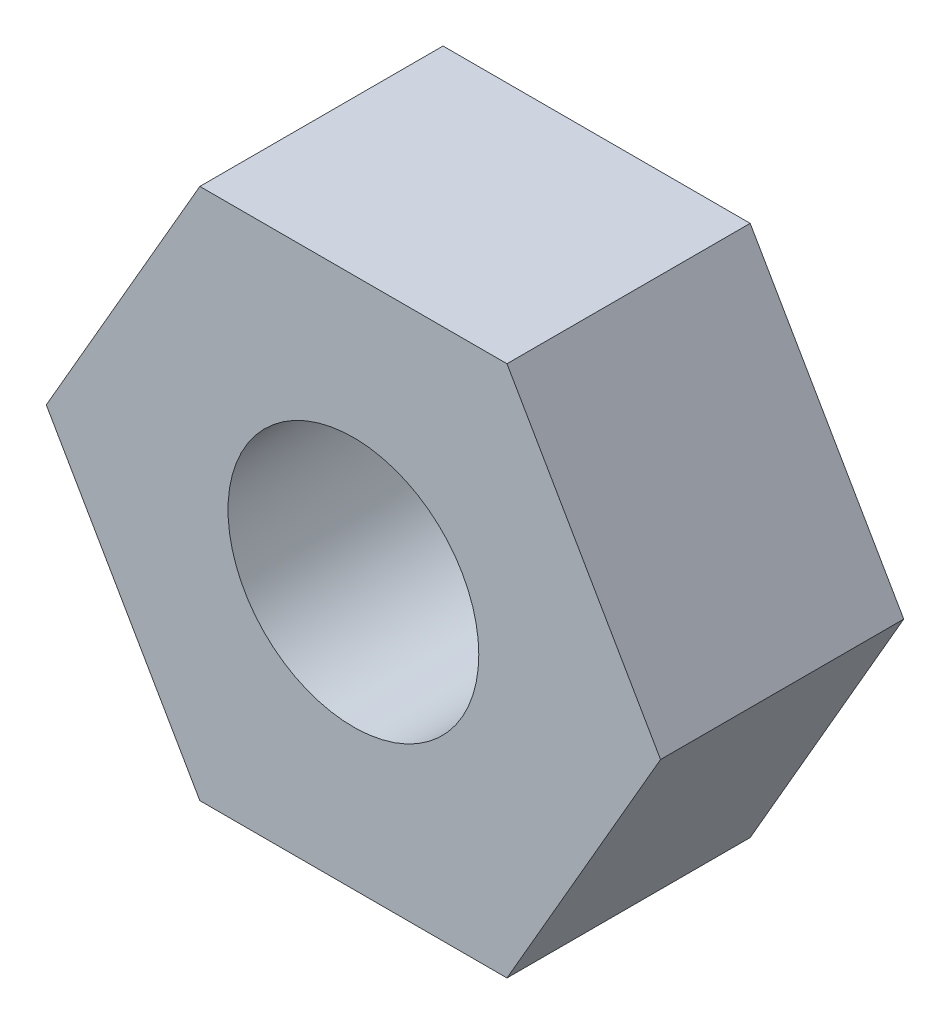
SolidWorks part; units mm, degrees
ref_plane "前视基准面" through (0, 0, 0) normal (0, 0, 1) x (1, 0, 0)
ref_plane "上视基准面" through (0, 0, 0) normal (0, 1, 0) x (1, 0, 0)
ref_plane "右视基准面" through (0, 0, 0) normal (1, 0, 0) x (0, 0, -1)
other "Configuration Table"
sketch "草图1" plane through (0, 0, 0) normal (0, 0, 1) x (1, 0, 0)
  line L0 (4.0415, 0) -> (2.0207, 3.5)
  line L1 (2.0207, 3.5) -> (-2.0207, 3.5)
  line L2 (-2.0207, 3.5) -> (-4.0415, 0)
  line L3 (-4.0415, 0) -> (-2.0207, -3.5)
  line L4 (-2.0207, -3.5) -> (2.0207, -3.5)
  line L5 (2.0207, -3.5) -> (4.0415, 0)
  circle A0 centre (0, 0) radius 1.65
  point P0 (0, 0)
  dimension "D1" = 3.3
  dimension "D2" = 2.0207
  dimension "D3" = 4.0415
  dimension "D4" = 6.0622
  dimension "D5" = 8.0829
  dimension "D6" = 3.5
  dimension "D7" = 7
extrude "凸台-拉伸1" add sketch "草图1" against normal mid plane 3.2
